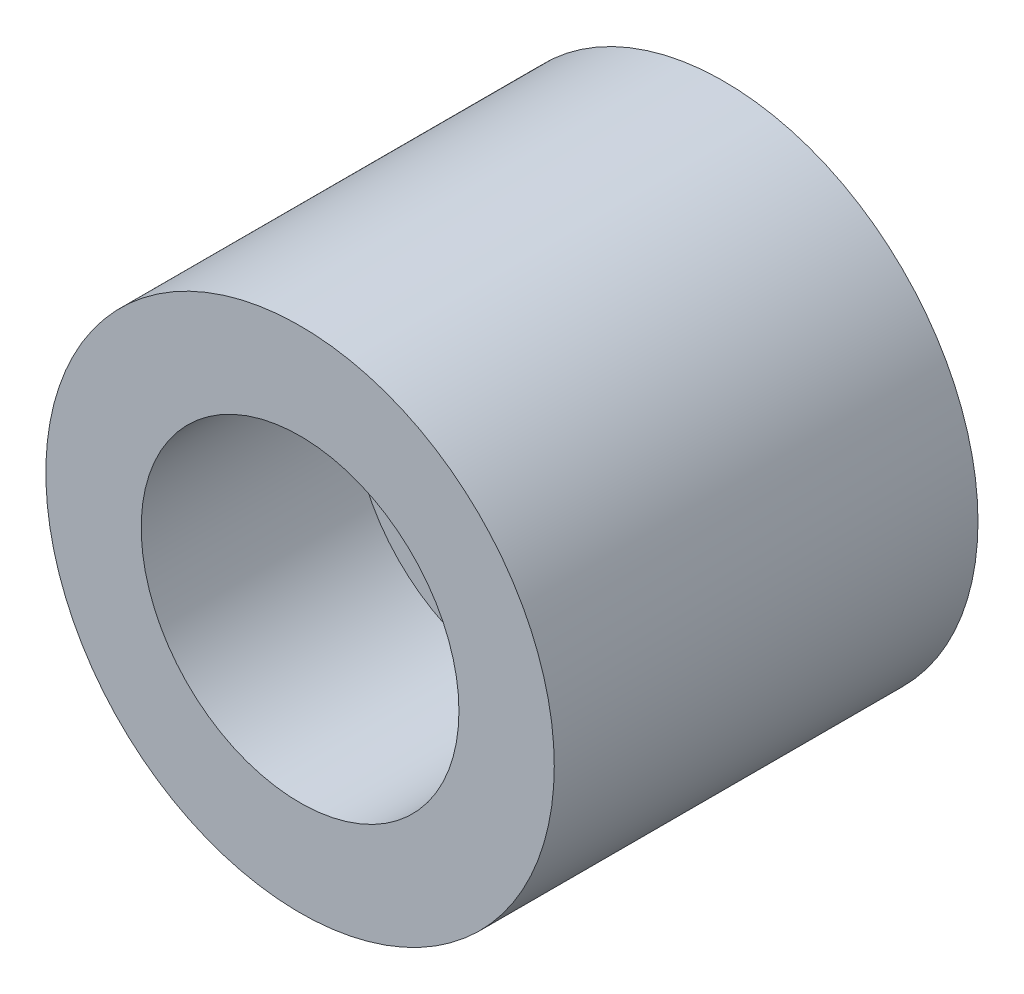
SolidWorks part; units mm, degrees
ref_plane "前视基准面" through (0, 0, 0) normal (0, 0, 1) x (1, 0, 0)
ref_plane "上视基准面" through (0, 0, 0) normal (0, 1, 0) x (1, 0, 0)
ref_plane "右视基准面" through (0, 0, 0) normal (1, 0, 0) x (0, 0, -1)
sketch "草图1" plane through (0, 0, 0) normal (0, 0, 1) x (1, 0, 0)
  circle A0 centre (0, 0) radius 6
  dimension "D1" = 12
extrude "凸台-拉伸1" add sketch "草图1" along normal blind 10
hole_wizard "打孔尺寸(%根据)内六角圆柱头螺钉的类型1" positions "草图2" profile "草图3" counterbore size "M4" standard "GB" end condition through all
sketch "草图2" plane through (0, 0, 10) normal (0, 0, 1) x (1, 0, 0)
  point P0 (0, 0)
sketch "草图3" plane through (0, 0, 10) normal (1, 0, 0) x (0, -1, 0)
  line L0 (0, 0) -> (0, 10)
  line L1 (0, 10) -> (2.25, 10)
  line L3 (2.25, 10) -> (2.25, 5)
  line L4 (2.25, 5) -> (3.75, 5)
  line L5 (3.75, 5) -> (3.75, 0)
  line L7 (3.75, 0) -> (0, 0)
  line L11 (0, -6.35) -> (0, 107.95) construction
  dimension "通孔孔直径" = 4.5
  dimension "通孔孔深度" = 10
  dimension "柱形沉头孔直径" = 7.5
  dimension "柱形沉头孔深度" = 5
